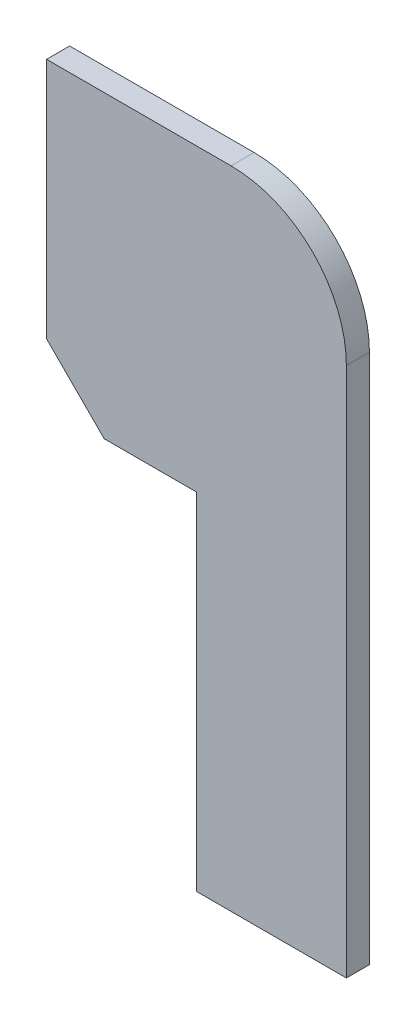
from build123d import *

# Parameters (mm, degrees)
BOSS_EXTRUDE1_DEPTH = 5


with BuildPart() as part:
    # Sketch1 → Boss-Extrude1 (new, symmetric)
    with BuildSketch(Plane.XY):
        with BuildLine():
            Line((0, 175), (0, 280))
            Line((0, 280), (80, 280))
            ThreePointArc((80, 280), (115.355339059, 265.355339059), (130, 230))
            Line((130, 230), (130, 0))
            Line((130, 0), (65, 0))
            Line((65, 0), (65, 150))
            Line((65, 150), (25, 150))
            Line((25, 150), (0, 175))
        make_face()
    extrude(amount=BOSS_EXTRUDE1_DEPTH, both=True)


solid = part.part
